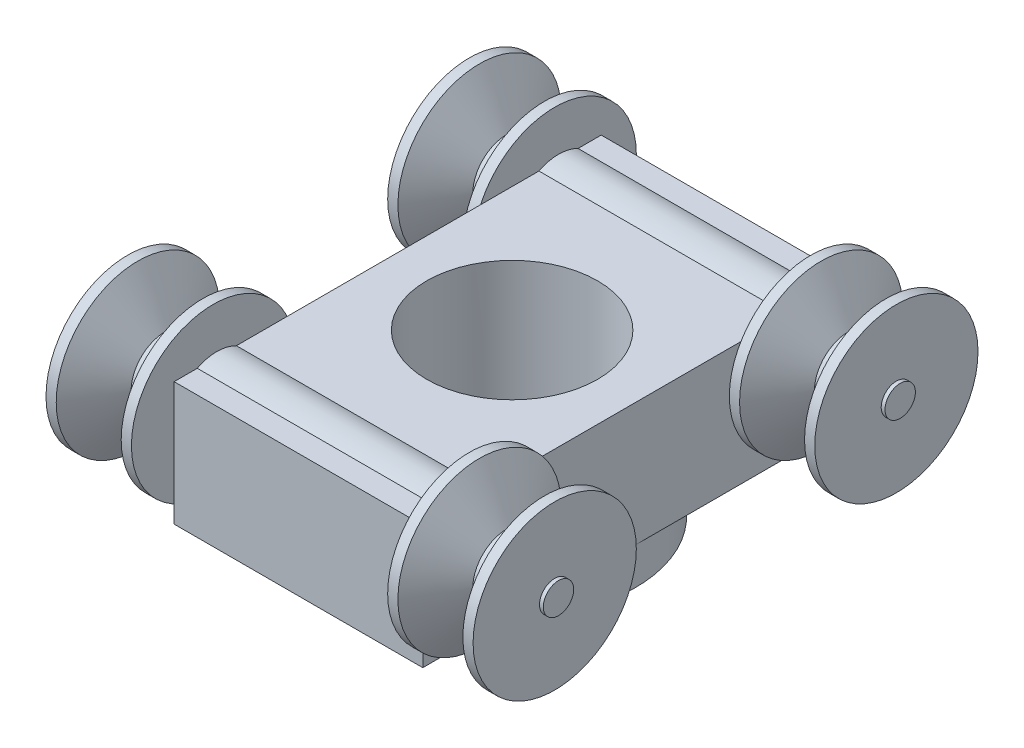
from build123d import *

# Parameters (mm, degrees)
LPATTERN1_COUNT          = 2
LPATTERN1_PITCH          = 180
SKETCH3_R                = 22.5
BOSS_EXTRUDE2_DEPTH      = 135
SKETCH4_R                = 30.412434653
SKETCH4_R_2              = 16
CUT_EXTRUDE1_DEPTH       = 2
SKETCH5_R                = 8
BOSS_EXTRUDE3_DEPTH      = 47
LPATTERN2_COUNT          = 2
LPATTERN2_PITCH          = 180
BOSS_EXTRUDE4_DEPTH      = 20
BOSS_EXTRUDE4_DEPTH_BACK = 45
SKETCH6_W                = 131
SKETCH6_H                = 225
SKETCH7_R                = 65
BOSS_EXTRUDE5_DEPTH      = 20
CUT_EXTRUDE2_DEPTH       = 342.400058582
CUT_EXTRUDE2_DEPTH_BACK  = 342.400058582
SKETCH8_R                = 45


with BuildPart() as part:
    # Sketch2 → Revolve1 (revolve)
    with BuildSketch(Plane(origin=(0, 0, 0), x_dir=(1, 0, 0), z_dir=(0, 1, 0)), mode=Mode.PRIVATE) as revolve1_sk:
        Polygon((0, 0), (0, 35), (5.386751346, 35), (19.820508076, 10), (25.179491924, 10), (39.613248654, 35), (45, 35), (45, 0), align=None)
    revolve(revolve1_sk.sketch.rotate(Axis((10.892128266, 0, 8), (1, 0, 0)), 180), axis=Axis((10.892128266, 0, 8), (1, 0, 0)))


with BuildPart() as lpattern1_1:
    # LPattern1: pattern copy
    add(part.part.moved(Location(Vector(1, 0, 0) * (1 * LPATTERN1_PITCH))))


with BuildPart() as part_1:
    add(part.part)

    add(lpattern1_1.part)  # Boss-Extrude2 merges LPattern1_1
    # Sketch3 → Boss-Extrude2 (add)
    with BuildSketch(Plane(origin=(45, 0, 0), x_dir=(0, 0, -1), z_dir=(1, 0, 0))):
        with Locations(Location((-8, 0, 0), (0, 0, 180))):
            Circle(SKETCH3_R)
    extrude(amount=BOSS_EXTRUDE2_DEPTH)

    # Sketch4 → Cut-Extrude1 (cut)
    with BuildSketch(Plane(origin=(45, 0, 0), x_dir=(0, 0, -1), z_dir=(1, 0, 0))):
        with Locations((-8, 0)):
            Circle(SKETCH4_R)
        with Locations((-8, 0)):
            Circle(SKETCH4_R_2, mode=Mode.SUBTRACT)
    cut_extrude1 = extrude(amount=CUT_EXTRUDE1_DEPTH, mode=Mode.SUBTRACT)

    # Mirror1: Cut-Extrude1 across plane
    add(cut_extrude1.mirror(Plane.ZY.offset(-112.5)), mode=Mode.SUBTRACT)

    # Sketch5 → Boss-Extrude3 (add)
    with BuildSketch(Plane(origin=(180, 0, 0), x_dir=(0, 0, -1), z_dir=(1, 0, 0))):
        with Locations(Location((-8, 0, 0), (0, 0, 180))):
            Circle(SKETCH5_R)
    boss_extrude3 = extrude(amount=BOSS_EXTRUDE3_DEPTH)

    # Mirror2: Boss-Extrude3 across plane
    add(boss_extrude3.mirror(Plane.ZY.offset(-112.5)))


with BuildPart() as lpattern2_1:
    # LPattern2: pattern copy
    add(part_1.part.moved(Location(Vector(0, 0, 1) * (1 * LPATTERN2_PITCH))))


with BuildPart() as part_2:
    add(part_1.part)

    add(lpattern2_1.part)  # Boss-Extrude4 merges LPattern2_1
    # Sketch6 → Boss-Extrude4 (add, two sides: drawn at the far end of the back side and taken through both)
    with BuildSketch(Plane(origin=(0, 0, 0), x_dir=(1, 0, 0), z_dir=(0, 1, 0)).offset(-BOSS_EXTRUDE4_DEPTH_BACK)):
        with Locations((112.5, -98)):
            Rectangle(SKETCH6_W, SKETCH6_H)
    extrude(amount=BOSS_EXTRUDE4_DEPTH + BOSS_EXTRUDE4_DEPTH_BACK)

    # Sketch7 → Boss-Extrude5 (add)
    with BuildSketch(Plane.XZ.offset(45)):
        with Locations(Location((112.5, 97.931490015, 0), (0, 0, 270))):
            Circle(SKETCH7_R)
    extrude(amount=BOSS_EXTRUDE5_DEPTH)

    # Sketch8 → Cut-Extrude2 (cut, two sides: drawn at the far end of the back side and taken through both)
    with BuildSketch(Plane.XZ.offset(65).offset(-CUT_EXTRUDE2_DEPTH_BACK)):
        with Locations(Location((112.5, 97.931490015, 0), (0, 0, 270))):
            Circle(SKETCH8_R)
    extrude(amount=CUT_EXTRUDE2_DEPTH + CUT_EXTRUDE2_DEPTH_BACK, mode=Mode.SUBTRACT)


solid = part_2.part
